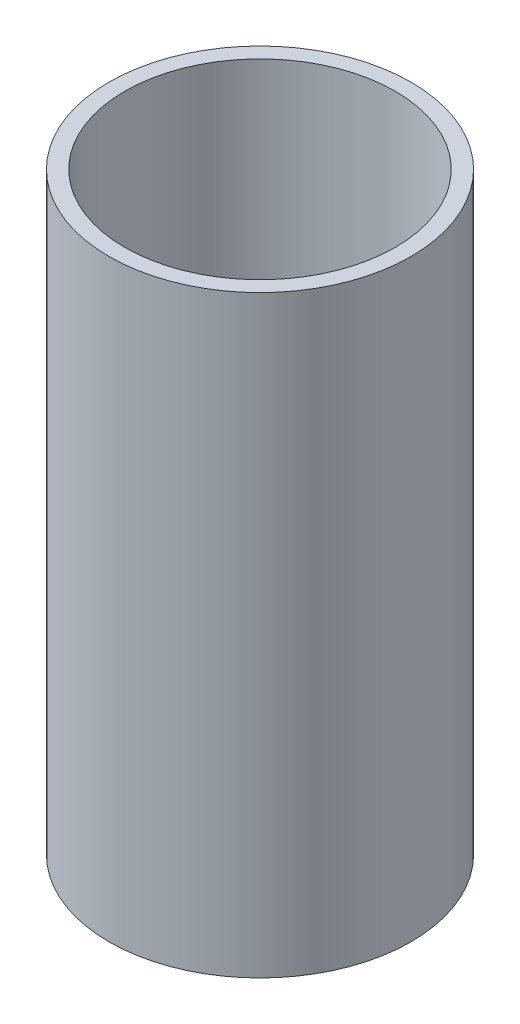
SolidWorks part; units mm, degrees
ref_plane "Front Plane" through (0, 0, 0) normal (0, 0, 1) x (1, 0, 0)
ref_plane "Top Plane" through (0, 0, 0) normal (0, 1, 0) x (1, 0, 0)
ref_plane "Right Plane" through (0, 0, 0) normal (1, 0, 0) x (0, 0, -1)
sketch "Sketch1" plane through (0, 0, 0) normal (0, 1, 0) x (1, 0, 0)
  circle A0 centre (0, 0) radius 11.5
  dimension "D1" = 23
extrude "Boss-Extrude1" add sketch "Sketch1" along normal blind 45.2
sketch "Sketch4" plane through (0, 45.2, 0) normal (0, 1, 0) x (1, 0, 0)
  circle A2 centre (0, 0) radius 10.3
  circle A3 centre (0, 0) radius 10.3
  dimension "D1" = 1.2
extrude "Cut-Extrude1" cut sketch "Sketch4" against normal blind 44
sketch "Sketch5" plane through (0, 0, 0) normal (0, -1, 0) x (1, 0, 0)
  circle A2 centre (0, 0) radius 9.8
  circle A3 centre (0, 0) radius 9.8
  dimension "D1" = 1.7
extrude "Cut-Extrude2" cut sketch "Sketch5" against normal blind 0.9
shell "Shell1" [suppressed] thickness 1
ref_plane "Plane1" [suppressed] through (0, 1.1, 0) normal (0, 1, 0) x (1, 0, 0)
sketch "Sketch3" [suppressed] plane through (0, 1.1, 0) normal (0, 1, 0) x (1, 0, 0)
  circle A0 centre (0, 0) radius 10.45
  dimension "D1" = 20.9
extrude "Boss-Extrude2" [suppressed] add sketch "Sketch3" along normal blind 40 separate body
dome "Dome1" [suppressed] faces to dome 2 distance 1 parameters "D1"=1
sketch "Sketch7" plane through (0, 1.2, 0) normal (0, 1, 0) x (1, 0, 0)
  circle A0 centre (0, 0) radius 10
  dimension "D1" = 20
extrude "Boss-Extrude3" [suppressed] add sketch "Sketch7" along normal blind 40
